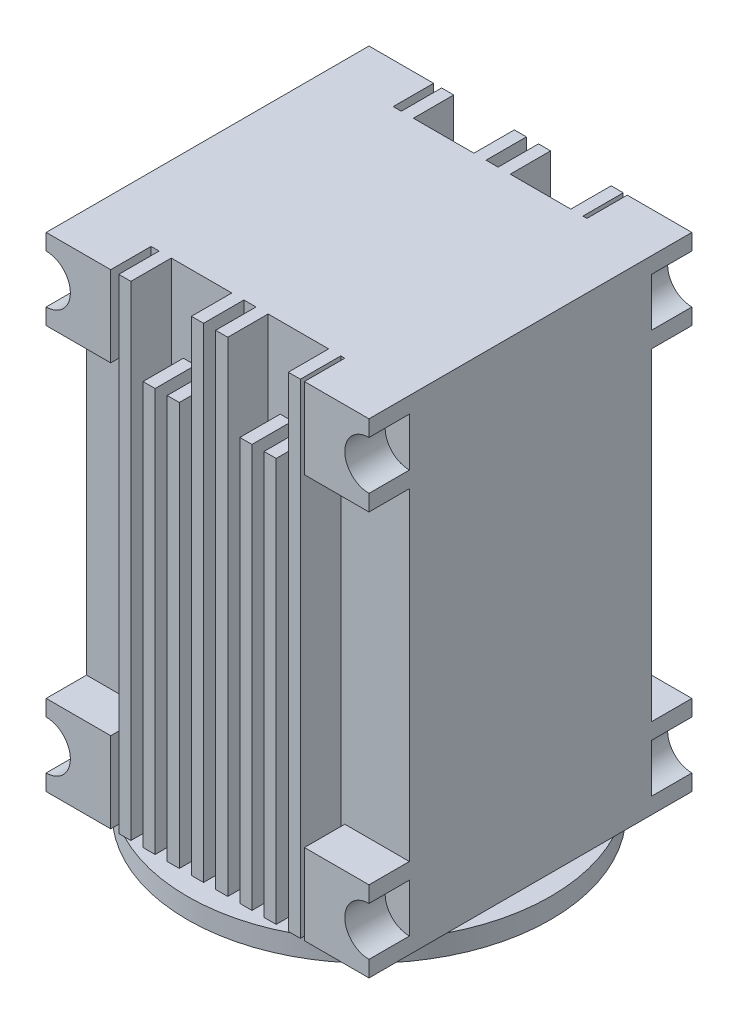
SolidWorks part; units mm, degrees
ref_plane "Front Plane" through (0, 0, 0) normal (0, 0, 1) x (1, 0, 0)
ref_plane "Top Plane" through (0, 0, 0) normal (0, 1, 0) x (1, 0, 0)
ref_plane "Right Plane" through (0, 0, 0) normal (1, 0, 0) x (0, 0, -1)
other "Configuration Table"
sketch "Sketch1" plane through (0, 0, 0) normal (0, 1, 0) x (1, 0, 0)
  line L1 (-20, -20) -> (20, -20)
  line L2 (-20, -20) -> (-20, 20)
  line L3 (-20, 20) -> (20, 20)
  line L4 (20, -20) -> (20, 20)
  line L5 (-20, -20) -> (20, 20) construction
  line L6 (-20, 20) -> (20, -20) construction
  point P0 (0, 0)
  dimension "D1" = 40
  dimension "D2" = 40
extrude "Boss-Extrude1" add sketch "Sketch1" along normal mid plane 60
sketch "Sketch2" plane through (0, 0, -20) normal (0, 0, -1) x (-1, 0, 0)
  line L0 (-12, 30) -> (12, 30)
  line L1 (-20, 30) -> (-12, 30) construction
  line L2 (-20, 30) -> (-20, 20) construction
  line L3 (-20, 20) -> (-12, 20)
  line L4 (-12, 30) -> (-12, 20)
  line L5 (20, 30) -> (12, 30) construction
  line L6 (20, 30) -> (20, 20) construction
  line L7 (20, 20) -> (12, 20)
  line L8 (12, 30) -> (12, 20)
  line L9 (-20, -30) -> (-12, -30) construction
  line L10 (-20, -30) -> (-20, -20) construction
  line L11 (-20, -20) -> (-12, -20)
  line L12 (-12, -30) -> (-12, -20)
  line L13 (20, -30) -> (12, -30) construction
  line L14 (20, -30) -> (20, -20) construction
  line L15 (20, -20) -> (12, -20)
  line L16 (12, -30) -> (12, -20)
  line L17 (-20, 20) -> (-20, -20)
  line L18 (-12, -30) -> (12, -30)
  line L19 (20, 20) -> (20, -20)
  dimension "D1" = 8
  dimension "D2" = 10
  dimension "D3" = 10
  dimension "D4" = 10
  dimension "D5" = 10
  dimension "D6" = 8
extrude "Cut-Extrude1" cut sketch "Sketch2" against normal blind 5
mirror "Mirror1" about plane through (0, 0, 0) normal (0, 0, 1) of "Cut-Extrude1"
sketch "Sketch3" plane through (0, 30, 0) normal (0, 1, 0) x (1, 0, 0)
  line L0 (-12, 15) -> (12, 15) construction
  line L1 (-11, 15) -> (-9.5, 15)
  line L2 (-11, 15) -> (-11, 20)
  line L3 (-11, 20) -> (-9.5, 20)
  line L4 (-9.5, 15) -> (-9.5, 20)
  line L5 (-12, 15) -> (-12, 20) construction
  line L6 (0, 0) -> (10.5943, 0) construction
  line L7 (-8, 20) -> (-6.5, 20)
  line L8 (-8, 15) -> (-8, 20)
  line L9 (-6.5, 15) -> (-6.5, 20)
  line L10 (-8, 15) -> (-6.5, 15)
  line L11 (-5, 20) -> (-3.5, 20)
  line L12 (-5, 15) -> (-5, 20)
  line L13 (-3.5, 15) -> (-3.5, 20)
  line L14 (-5, 15) -> (-3.5, 15)
  line L15 (-2, 20) -> (-0.5, 20)
  line L16 (-2, 15) -> (-2, 20)
  line L17 (-0.5, 15) -> (-0.5, 20)
  line L18 (-2, 15) -> (-0.5, 15)
  line L19 (1, 20) -> (2.5, 20)
  line L20 (1, 15) -> (1, 20)
  line L21 (2.5, 15) -> (2.5, 20)
  line L22 (1, 15) -> (2.5, 15)
  line L23 (4, 20) -> (5.5, 20)
  line L24 (4, 15) -> (4, 20)
  line L25 (5.5, 15) -> (5.5, 20)
  line L26 (4, 15) -> (5.5, 15)
  line L27 (7, 20) -> (8.5, 20)
  line L28 (7, 15) -> (7, 20)
  line L29 (8.5, 15) -> (8.5, 20)
  line L30 (7, 15) -> (8.5, 15)
  line L31 (10, 20) -> (11.5, 20)
  line L32 (10, 15) -> (10, 20)
  line L33 (11.5, 15) -> (11.5, 20)
  line L34 (10, 15) -> (11.5, 15)
  dimension "D1" = 1
  dimension "D2" = 1.5
  dimension "D4" = 3
  dimension "D3" = 8
extrude "Boss-Extrude2" add sketch "Sketch3" against normal up to surface (60 mm away) up to face at (0, -30, 0)
sketch "Sketch4" plane through (0, 0, -20) normal (0, 0, -1) x (-1, 0, 0)
  line L0 (-4, -30) -> (-4, 30) construction
  line L1 (-8.5, 30) -> (-4, 30)
  line L2 (-8.5, 30) -> (-8.5, 20)
  line L3 (-8.5, 20) -> (-4, 20)
  line L4 (-4, 30) -> (-4, 20)
  line L5 (8, -30) -> (8, 30) construction
  line L6 (3.5, 30) -> (8, 30)
  line L7 (3.5, 30) -> (3.5, 20)
  line L8 (3.5, 20) -> (8, 20)
  line L9 (8, 30) -> (8, 20)
  dimension "D1" = 10
extrude "Cut-Extrude2" cut sketch "Sketch4" against normal blind 5
mirror "Mirror2" about plane through (0, 0, 0) normal (0, 0, 1) of "Cut-Extrude2", "Boss-Extrude2"
sketch "Sketch5" plane through (0, 0, -20) normal (0, 0, -1) x (-1, 0, 0)
  line L0 (-20, 30) -> (-20, 20) construction
  line L2 (0, 0) -> (0, 10.117) construction
  line L3 (0, 0) -> (16.5103, 0) construction
  circle A1 centre (-20, 25) radius 3
  circle A2 centre (20, 25) radius 3
  circle A3 centre (-20, -25) radius 3
  circle A4 centre (20, -25) radius 3
  dimension "D1" = 6
extrude "Cut-Extrude3" cut sketch "Sketch5" against normal blind 5
mirror "Mirror3" about plane through (0, 0, 0) normal (0, 0, 1) of "Cut-Extrude3"
sketch "Sketch6" plane through (0, -30, 0) normal (0, -1, 0) x (1, 0, 0)
  circle A0 centre (0, 0) radius 22.5
  dimension "D1" = 45
extrude "Boss-Extrude3" add sketch "Sketch6" along normal blind 2.5 contours A0
sketch "Sketch7" plane through (0, -32.5, 0) normal (0, -1, 0) x (1, 0, 0)
  circle A0 centre (0, 0) radius 5
  dimension "D1" = 10
extrude "Cut-Extrude4" cut sketch "Sketch7" against normal blind 15 contours A0
sketch "Sketch8" plane through (-20, 0, 0) normal (-1, 0, 0) x (0, 0, 1)
  line L0 (-20, 30) -> (20, 30) construction
  circle A0 centre (-0.51, 13.59) radius 2.5
  dimension "D3" = 5
  dimension "D1" = 19.49
  dimension "D2" = 16.41
extrude "Cut-Extrude5" cut sketch "Sketch8" against normal blind 10 contours A0
sketch "Sketch9" plane through (0, -30, 0) normal (0, -1, 0) x (1, 0, 0)
  line L1 (-20, -20) -> (-20, -10.3078) construction
  line L2 (-12, -20) -> (-20, -20) construction
  line L3 (20, -10.3078) -> (20, -20) construction
  line L4 (12, 20) -> (20, 20) construction
  line L5 (-20, 20) -> (-12, 20) construction
  circle A0 centre (-17.5, 17.5) radius 1
  circle A1 centre (17.5, 17.5) radius 1
  circle A2 centre (17.5, -17.5) radius 1
  circle A3 centre (-17.5, -17.5) radius 1
  dimension "D1" = 2
  dimension "D4" = 2
  dimension "D8" = 2
  dimension "D9" = 2
  dimension "D2" = 2.5
  dimension "D3" = 2.5
  dimension "D5" = 2.5
  dimension "D6" = 2.5
  dimension "D7" = 2.5
extrude "Cut-Extrude6" cut sketch "Sketch9" against normal blind 1.8
